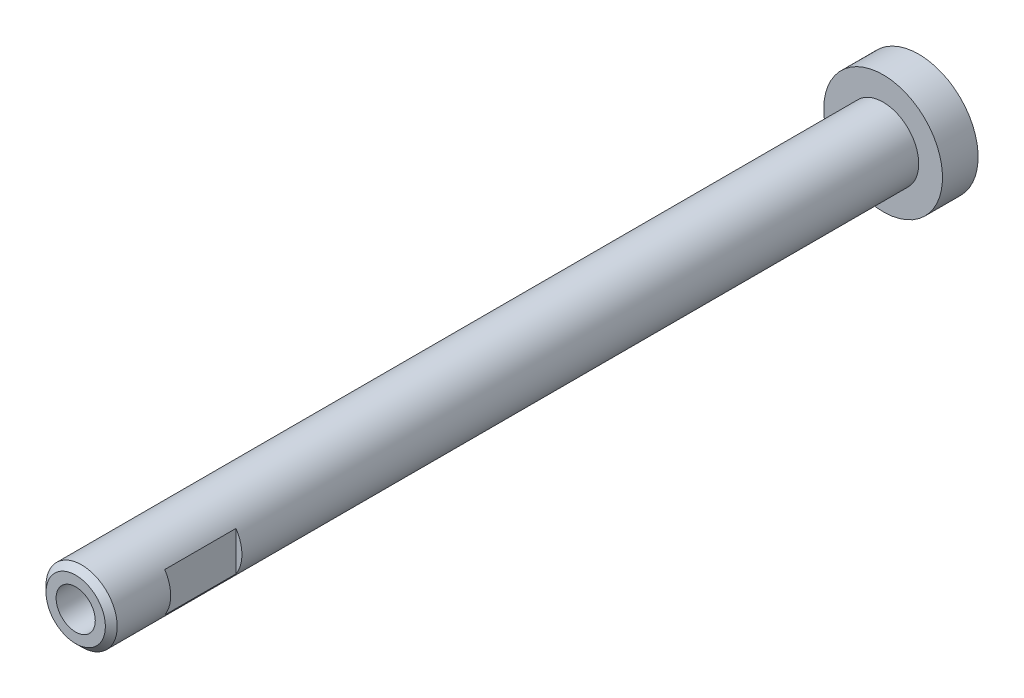
from build123d import *

# Parameters (mm, degrees)
SKETCH_1_R             = 3
EXTRUDE_1_DEPTH        = 71
HOLE_WIZARD_M4_2_D     = 3.3
HOLE_WIZARD_M4_2_DEPTH = 11.5
HOLE_WIZARD_M4_2_TIP   = 0.991420021
CHAMFER_1_SIZE         = 0.5
EXTRUDE1_DEPTH         = 72.126647608
EXTRUDE1_DEPTH_BACK    = 72.126647608
SKETCH1_W              = 2.697137816
SKETCH1_H              = 6
SKETCH1_W_2            = 2.361838602
SKETCH4_R              = 5
SKETCH4_R_2            = 3
EXTRUDE2_DEPTH         = 3


with BuildPart() as part:
    # 草图1 → 凸台-拉伸1 (new body)
    with BuildSketch(Plane.XY):
        Circle(SKETCH_1_R)
    extrude(amount=EXTRUDE_1_DEPTH)

    # M4 螺纹孔2
    with Locations(Plane.XY.offset(71)):
        with Locations((0, 0)):
            Hole(HOLE_WIZARD_M4_2_D / 2, depth=HOLE_WIZARD_M4_2_DEPTH)
            with Locations((0, 0, -(HOLE_WIZARD_M4_2_DEPTH + HOLE_WIZARD_M4_2_TIP / 2))):  # 118° drill point
                Cone(0, HOLE_WIZARD_M4_2_D / 2, HOLE_WIZARD_M4_2_TIP, mode=Mode.SUBTRACT)

    # 倒角1
    chamfer_1_edges = [part.edges().sort_by_distance(p)[0] for p in [
        (-3, 0, 71),
    ]]
    chamfer(chamfer_1_edges, length=CHAMFER_1_SIZE)

    # Sketch1 → Extrude1 (cut, two sides: drawn at the far end of the back side and taken through both)
    with BuildSketch(Plane(origin=(0, 0, 0), x_dir=(1, 0, 0), z_dir=(0, 1, 0)).offset(-EXTRUDE1_DEPTH_BACK)):
        with Locations((-3.848568908, -63)):
            Rectangle(SKETCH1_W, SKETCH1_H)
        with Locations((3.680919301, -63)):
            Rectangle(SKETCH1_W_2, SKETCH1_H)
    extrude(amount=EXTRUDE1_DEPTH + EXTRUDE1_DEPTH_BACK, mode=Mode.SUBTRACT)

    # Sketch4 → Extrude2 (add)
    with BuildSketch(Plane(origin=(0, 0, 0), x_dir=(-1, 0, 0), z_dir=(0, 0, -1))):
        Circle(SKETCH4_R)
        Circle(SKETCH4_R_2, mode=Mode.SUBTRACT)
    extrude(amount=-EXTRUDE2_DEPTH)


solid = part.part
